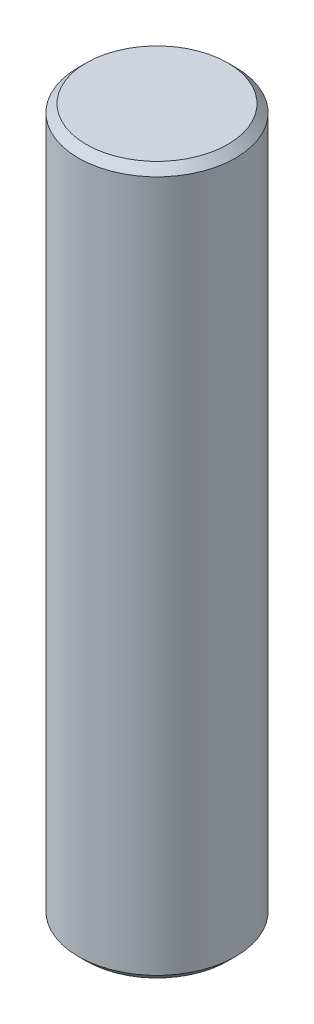
from build123d import *

# Parameters (mm, degrees)
SKETCH1_R             = 5
BOSS_EXTRUDE1_DEPTH   = 45
M5_TAPPED_HOLE1_D     = 4.2
M5_TAPPED_HOLE1_DEPTH = 12.4
M5_TAPPED_HOLE1_TIP   = 1.2618073
CHAMFER1_SIZE         = 0.5


with BuildPart() as part:
    # Sketch1 → Boss-Extrude1 (new body)
    with BuildSketch(Plane(origin=(0, 0, 0), x_dir=(1, 0, 0), z_dir=(0, 1, 0))):
        with Locations(Location((0, 0, 0), (0, 0, 90))):
            Circle(SKETCH1_R)
    extrude(amount=BOSS_EXTRUDE1_DEPTH)

    # M5 Tapped Hole1
    with Locations(Plane(origin=(0, 0, 0), x_dir=(0, 0, -1), z_dir=(0, -1, 0))):
        with Locations((0, 0)):
            Hole(M5_TAPPED_HOLE1_D / 2, depth=M5_TAPPED_HOLE1_DEPTH)
            with Locations((0, 0, -(M5_TAPPED_HOLE1_DEPTH + M5_TAPPED_HOLE1_TIP / 2))):  # 118° drill point
                Cone(0, M5_TAPPED_HOLE1_D / 2, M5_TAPPED_HOLE1_TIP, mode=Mode.SUBTRACT)

    # Chamfer1
    chamfer1_edges = [part.edges().sort_by_distance(p)[0] for p in [
        (0, 0, 5),
        (0, 45, 5),
    ]]
    chamfer(chamfer1_edges, length=CHAMFER1_SIZE)


solid = part.part
